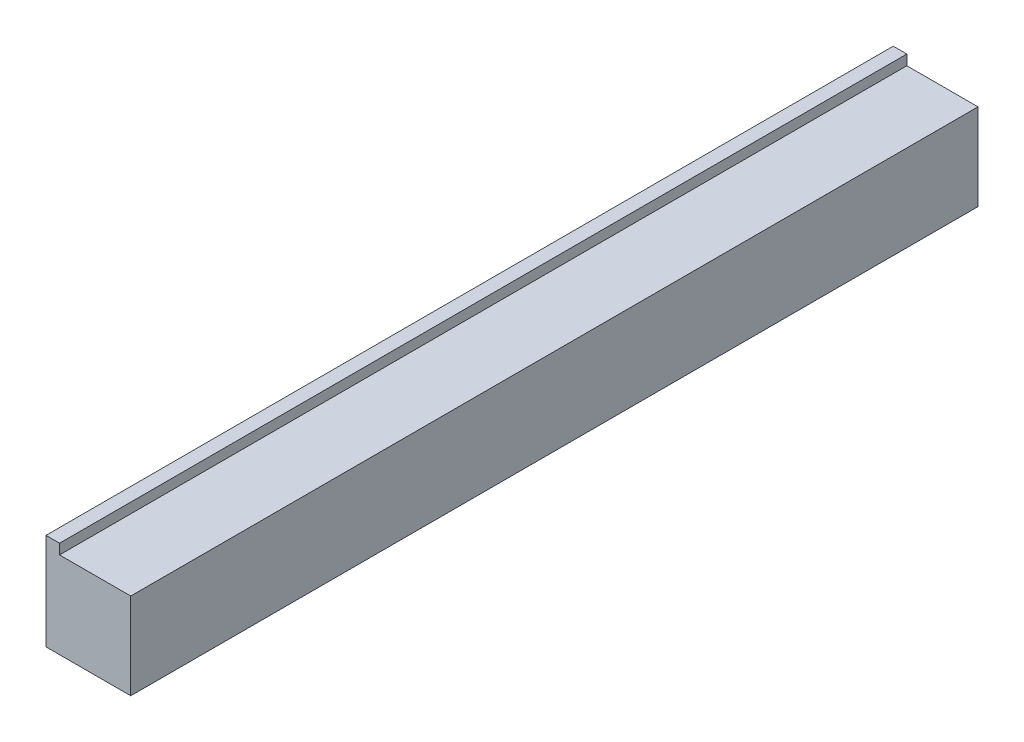
from build123d import *

# Parameters (mm, degrees)
EXTRUDE_1_DEPTH = 250


with BuildPart() as part:
    # 草图1 → 凸台-拉伸1 (new body)
    with BuildSketch(Plane.XY):
        Polygon((-10, -12.5), (-14, -12.5), (-14, -41), (11, -41), (11, -15.5), (-10, -15.5), align=None)
    extrude(amount=-EXTRUDE_1_DEPTH)


solid = part.part
